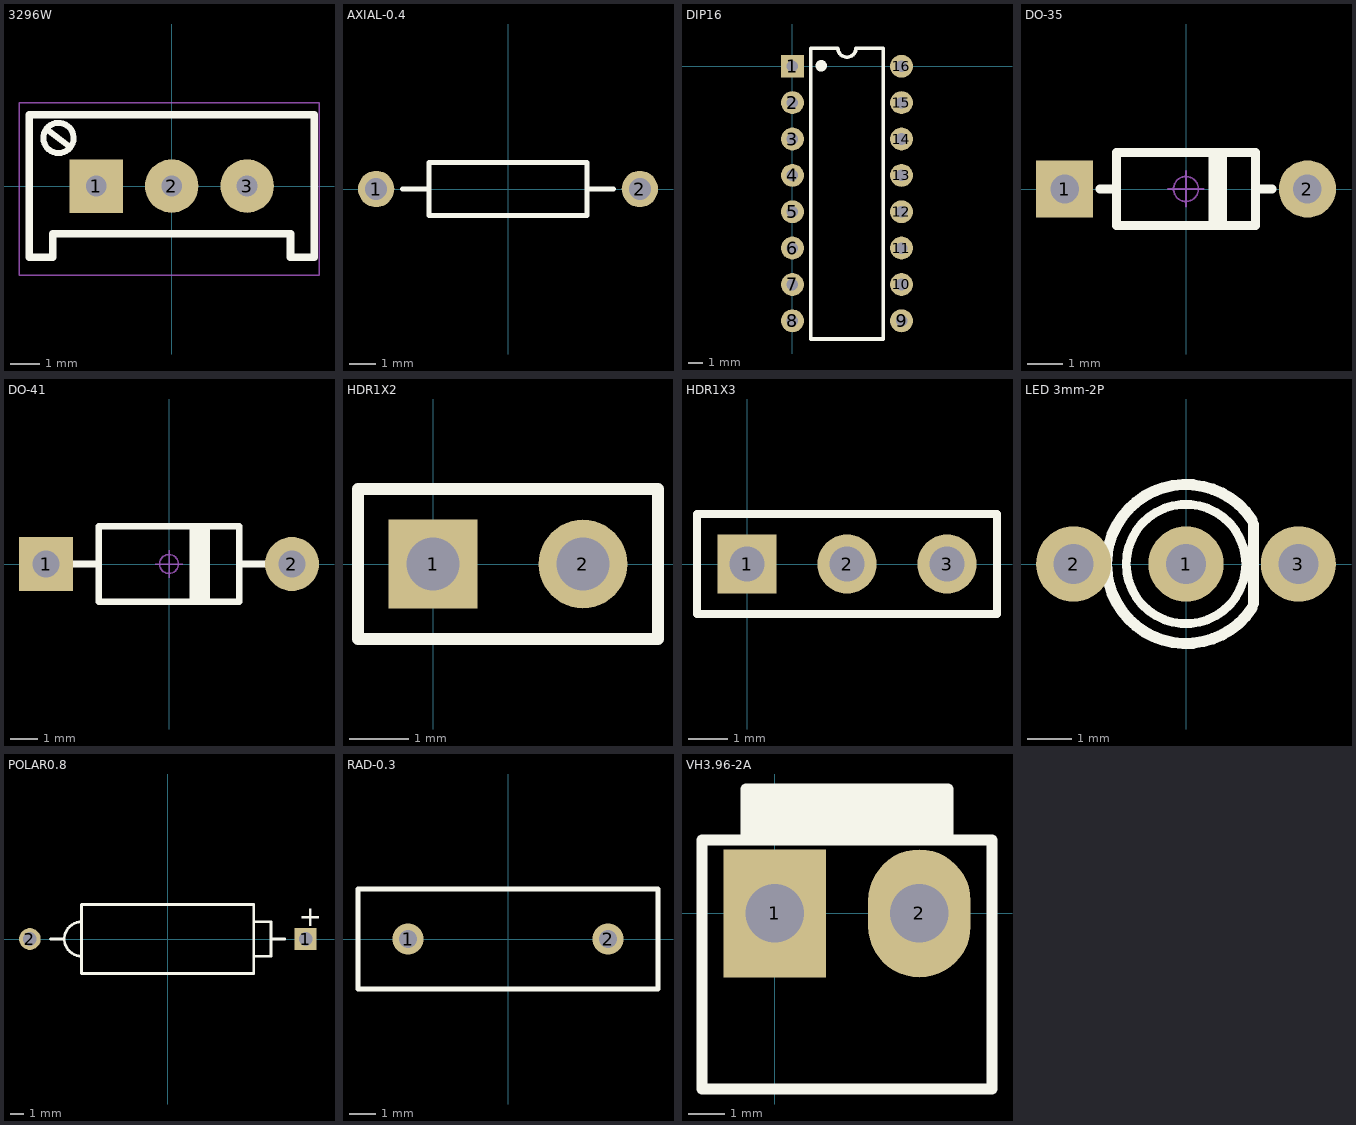
[diagram p0: the footprints below, top view; thin cyan lines are the x and y axes]
# Altium footprint library MISC82068.PcbLib: 11 footprints
Each footprint in its own frame and in the unit in brackets; x right, y up, seen from the top. Pads: shape width x height; smd on the part's side, far side on the other; paste and mask are expansions set on the pad; w line width, h text height; cw(c..) or ccw(c..) is an arc to the next point about the centre after c.

## 3296W [mm] "Precise Multi-Winding Adjustable Resistor"
height 4.58
pads (3):
  rect 1.8x1.8 hole 0.7: 1(-2.54,0)
  round 1.8 hole 0.7: 2(0,0) 3(2.54,0)
Top Overlay:
  lines w0.2: -3.302,1.651 ccw(c-3.81,1.618) -3.301,1.608
  lines w0.203: -4.2,1.9 -3.464,1.348
  lines w0.254: -4.8,-2.4 -4.8,2.4 4.8,2.4 4.8,-2.4 4,-2.4 4,-1.6 -4,-1.6 -4,-2.4 -4.8,-2.4
Mechanical 15:
  lines w0.05: -5.14,-3 4.96,-3 4.96,2.8 -5.14,2.8 -5.14,-3
3D body "3296.STEP": height 11.52, standoff -3.48, extent -4.75,-2.4 4.75,2.4

## AXIAL-0.4 [mm] "Axial Device, Thru-Hole; 2 Leads; 0.4 in Pin Spacing"
height 2.032
pads (2):
  round 1.4 hole 0.85: 1(-5.08,0) 2(5.08,0)
Top Overlay:
  lines w0.2: -4.064,0 -3.048,0 ; 3.048,0 4.064,0 ; -3.048,-1.016 -3.048,1.016 3.048,1.016 3.048,-1.016 -3.048,-1.016

## DIP16 [mm]
height 4.58
pads (16):
  rect 1.6x1.6 hole 0.813: 1(0,0)
  round 1.6 hole 0.813: 2(0,-2.54) 3(0,-5.08) 4(0,-7.62) 5(0,-10.16) 6(0,-12.7) 7(0,-15.24) 8(0,-17.78) 9(7.627,-17.78) 10(7.62,-15.24) 11(7.62,-12.7) 12(7.62,-10.16) 13(7.62,-7.62) 14(7.62,-5.08) 15(7.62,-2.54) 16(7.62,0)
Top Overlay:
  circle w0.5: c2.014,0.035 r0.15
  lines w0.254: 1.27,-19.05 6.35,-19.05 6.35,1.27 4.445,1.27 cw(c3.81,1.27) 3.175,1.27 1.27,1.27 1.27,-19.05
3D body "DIP16.STEP": height 5.1, standoff -3.3, extent -0.119,-18.763 7.751,1.237

## DO-35 [mm] "1.8*6.8mm (diameter, lead spacing)"
height 4.58
pads (2):
  rect 1.6x1.6 hole 0.8: 1(-3.4,0)
  round 1.6 hole 0.8: 2(3.4,0)
Top Overlay:
  rectangle: 0.635,-1.016 1.143,1.016
  lines w0.254: -2.413,0 -1.95,0 ; 1.95,0 2.413,0 ; -1.95,-1.016 1.95,-1.016 1.95,1.016 -1.95,1.016 -1.95,-1.016
Mechanical 15:
  circle w0.05: c0,0 r0.35
  lines w0.05: -0.5,0 0.5,0 ; 0,-0.5 0,0.5
3D body "DO-35.STEP": height 1.85, standoff -3.45, extent -3.65,-0.901 3.65,0.901

## DO-41 [mm] "2.6*9.1mm (diameter, lead spacing)"
height 2.4
pads (2):
  rect 2x2 hole 1: 1(-4.55,0)
  round 2 hole 1: 2(4.55,0)
Top Overlay:
  rectangle: 0.762,-1.397 1.524,1.397
  lines w0.254: -3.556,0 -2.6,0 ; 2.6,0 3.556,0 ; -2.6,-1.397 2.6,-1.397 2.6,1.397 -2.6,1.397 -2.6,-1.397
Mechanical 15:
  circle w0.05: c0,0 r0.35
  lines w0.05: -0.5,0 0.5,0 ; 0,-0.5 0,0.5
3D body "DO-41.STEP": height 2.65, standoff -3.45, extent -4.925,-1.288 4.975,1.314

## HDR1X2 [mm] "Connector; Header; 2 Position"
height 4.58
pads (2):
  rect 1.5x1.5 hole 0.9: 1(0,0)
  round 1.5 hole 0.9: 2(2.54,0)
Top Overlay:
  lines w0.2: -1.27,-1.27 3.81,-1.27 3.81,1.27 -1.27,1.27 -1.27,-1.27

## HDR1X3 [mm] "Connector; Header; 3 Position"
height 4.58
pads (3):
  rect 1.5x1.5 hole 0.9: 1(0,0)
  round 1.5 hole 0.9: 2(2.54,0) 3(5.08,0)
Top Overlay:
  lines w0.2: -1.27,-1.27 6.35,-1.27 6.35,1.27 -1.27,1.27 -1.27,-1.27

## LED 3mm-2P [mm] "3mm bicolour LED"
height 5
pads (3):
  round 1.7 hole 0.9: 1(0,0) 2(-2.54,0) 3(2.54,0)
Top Overlay:
  circle w0.2: c0,0 r1.35
  lines w0.254: 1.494,-0.996 cw(c0,0) 1.494,0.996 ; 1.524,-0.889 1.524,0.889
3D body "3MM ˫ɫLED.STEP": height 3.82, standoff -3.15, extent -2.79,-0.75 2.79,0.75
3D body "3MM 双色LED-灯罩.STEP": height 6.9, standoff 1.4, extent -1.95,-1.95 1.696,1.95

## POLAR0.8 [mm] "Polarized Capacitor; 2 Leads"
height 5.08
pads (2):
  rect 1.6x1.6 hole 1: 1(10.16,0)
  round 1.6 hole 1: 2(-10.16,0)
Top Overlay:
  lines w0.2: -8.636,0 -7.62,0 ; -6.35,-1.27 cw(c-6.35,0) -6.35,1.27 ; 6.35,-1.27 7.62,-1.27 7.62,1.27 6.35,1.27 ; 7.62,0 8.636,0 ; -6.35,-2.54 -6.35,2.54 6.35,2.54 6.35,-2.54 -6.35,-2.54
  text "+" at 9.652,0.95 h1.5

## RAD-0.3 [mm] "Radial Cap, Thru-Hole; 2 Leads; 0.3 in Pin Spacing"
height 6
pads (2):
  round 1.2 hole 0.7: 1(-3.81,0) 2(3.81,0)
Top Overlay:
  lines w0.2: -5.715,-1.905 5.715,-1.905 5.715,1.905 -5.715,1.905 -5.715,-1.905

## VH3.96-2A [mm]
height 4.58
pads (2):
  rect 2.8x3.5 hole 1.6: 1(0,0)
  oval 2.8x3.5 hole 1.6: 2(3.96,0)
Top Overlay:
  lines w0.3: -0.78,2 -0.78,3.4 4.74,3.4 4.74,2 ; -0.78,2.286 4.74,2.286 ; -0.78,2.413 4.74,2.413 ; -0.78,2.667 4.74,2.667 ; -0.78,2.921 4.74,2.921 ; -0.78,3.175 4.74,3.175 ; -1.98,-4.8 -1.98,2 5.94,2 5.94,-4.8 -1.98,-4.8
3D body "VH3.96-2A.STEP": height 14.6, standoff -3.6, extent -1.98,-4.8 5.94,3.6